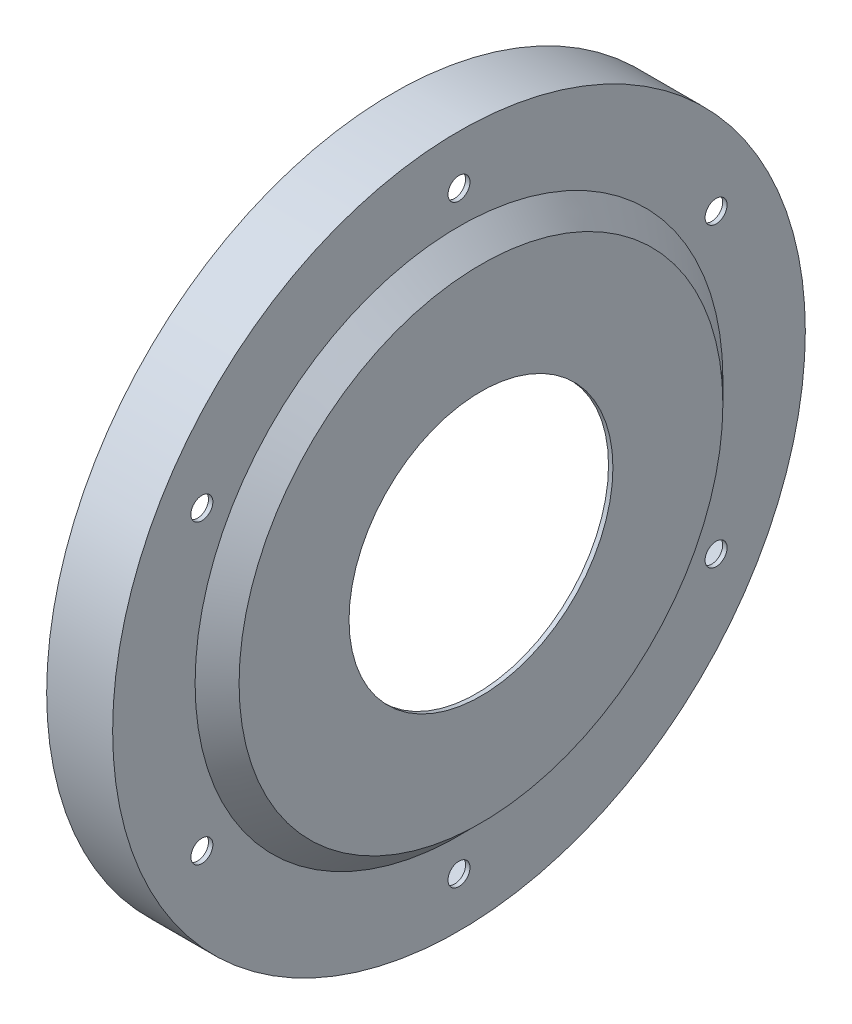
from build123d import *

# Parameters (mm, degrees)
SHELL1_T           = -2
SKETCH2_R          = 60
CUT_EXTRUDE1_DEPTH = 50
SKETCH3_R          = 5
CUT_EXTRUDE2_DEPTH = 50


with BuildPart() as part:
    # Sketch1 → Revolve1 (revolve)
    with BuildSketch(Plane(origin=(0, 0, 0), x_dir=(1, 0, 0), z_dir=(0, 1, 0)), mode=Mode.PRIVATE) as revolve1_sk:
        Polygon((0, 0), (0, 157.5), (30, 157.5), (30, 120), (40, 110), (40, 0), align=None)
    revolve(revolve1_sk.sketch.rotate(Axis((0, 0, 0), (1, 0, 0)), 180), axis=Axis((0, 0, 0), (1, 0, 0)))

    # Shell1
    shell1_openings = [part.faces().sort_by_distance(p)[0] for p in [
        (0, 0, 0),
    ]]
    offset(amount=SHELL1_T, openings=shell1_openings, kind=Kind.INTERSECTION)

    # Sketch2 → Cut-Extrude1 (cut)
    with BuildSketch(Plane(origin=(40, 0, 0), x_dir=(0, 0, -1), z_dir=(1, 0, 0))):
        Circle(SKETCH2_R)
    extrude(amount=-CUT_EXTRUDE1_DEPTH, mode=Mode.SUBTRACT)

    # Sketch3 → Cut-Extrude2 (cut)
    with BuildSketch(Plane(origin=(30, 0, 0), x_dir=(0, 0, -1), z_dir=(1, 0, 0))):
        with Locations((0, 135)):
            Circle(SKETCH3_R)
        with Locations((116.913429511, 67.5)):
            Circle(SKETCH3_R)
        with Locations((116.913429511, -67.5)):
            Circle(SKETCH3_R)
        with Locations((0, -135)):
            Circle(SKETCH3_R)
        with Locations((-116.913429511, -67.5)):
            Circle(SKETCH3_R)
        with Locations((-116.913429511, 67.5)):
            Circle(SKETCH3_R)
    extrude(amount=-CUT_EXTRUDE2_DEPTH, mode=Mode.SUBTRACT)


solid = part.part
